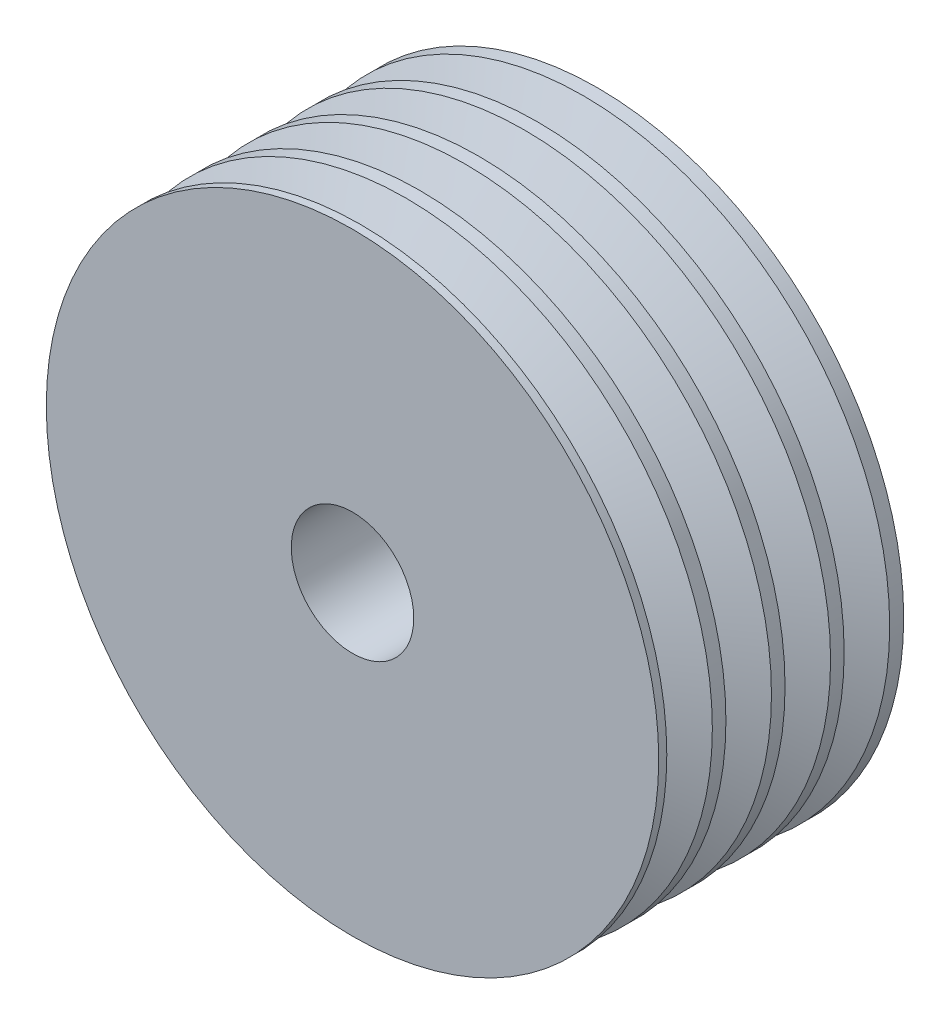
from build123d import *

# Parameters (mm, degrees)
SKETCH_1_R      = 75
SKETCH_1_R_2    = 15
EXTRUDE_1_DEPTH = 60


with BuildPart() as part:
    # 草图1 → 凸台-拉伸1 (new body)
    with BuildSketch(Plane.XY):
        Circle(SKETCH_1_R)
        Circle(SKETCH_1_R_2, mode=Mode.SUBTRACT)
    extrude(amount=EXTRUDE_1_DEPTH)

    # 草图2 → 切除-旋转2 (revolve, cut)
    with BuildSketch(Plane(origin=(0, 0, 0), x_dir=(1, 0, 0), z_dir=(0, 1, 0)), mode=Mode.PRIVATE) as cut_revolve_2_sk:
        Polygon((-75, -46.866291189), (-75, -58.022292434), (-64.263367228, -52.307244529), (-64.263367228, -51.572801228), align=None)
        Polygon((-75, -32.38659394), (-75, -43.542595186), (-64.263367228, -37.827547281), (-64.263367228, -37.09310398), align=None)
        Polygon((-75, -17.906896692), (-75, -29.062897938), (-64.263367228, -23.347850033), (-64.263367228, -22.613406731), align=None)
        Polygon((-75, -3.427199444), (-75, -14.583200689), (-64.263367228, -8.868152785), (-64.263367228, -8.133709483), align=None)
    revolve(cut_revolve_2_sk.sketch.rotate(Axis((0, 0, 0), (0, 0, -1)), 180), axis=Axis((0, 0, 0), (0, 0, -1)), mode=Mode.SUBTRACT)


solid = part.part
